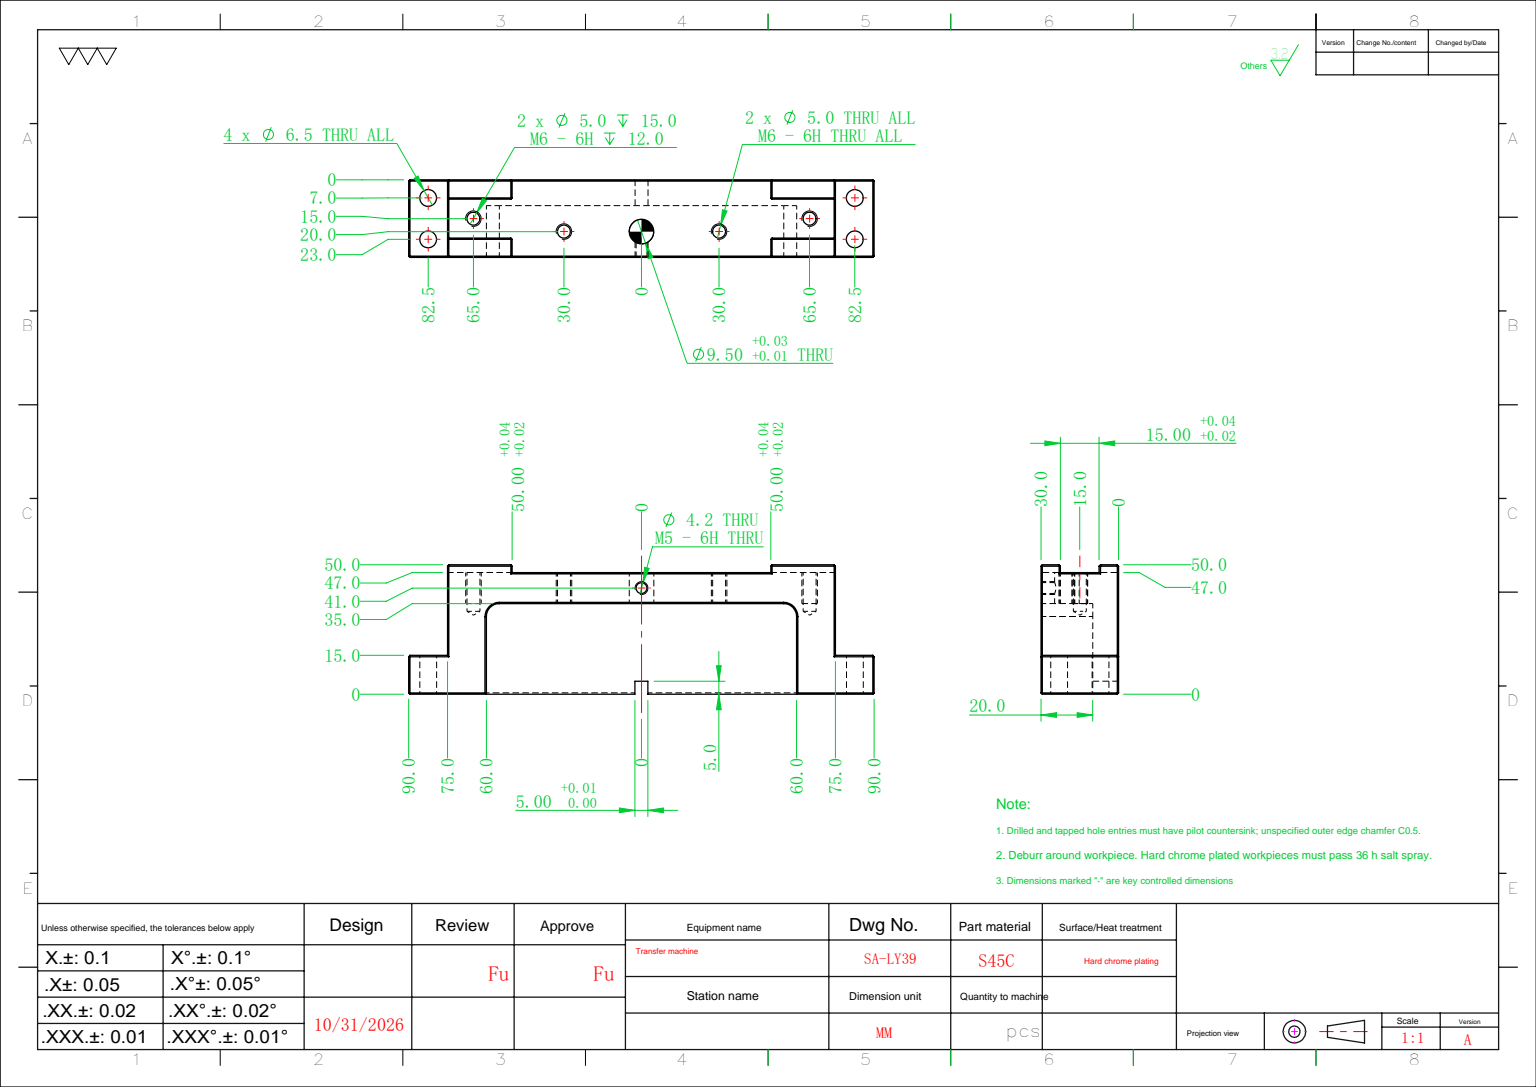
SolidWorks part; units mm, degrees
ref_plane "前视基准面" through (0, 0, 0) normal (0, 0, 1) x (1, 0, 0)
ref_plane "上视基准面" through (0, 0, 0) normal (0, 1, 0) x (1, 0, 0)
ref_plane "右视基准面" through (0, 0, 0) normal (1, 0, 0) x (0, 0, -1)
sketch "草图1" plane through (0, 0, 0) normal (0, 0, 1) x (1, 0, 0)
  line L1 (-75, -15) -> (75, -15)
  line L2 (-75, -15) -> (-75, 15)
  line L3 (-75, 15) -> (75, 15)
  line L4 (75, -15) -> (75, 15)
  line L5 (-75, -15) -> (75, 15) construction
  line L6 (-75, 15) -> (75, -15) construction
  point P0 (0, 0)
  dimension "D1" = 150
  dimension "D2" = 30
extrude "凸台-拉伸1" add sketch "草图1" along normal blind 50
sketch "草图3" plane through (0, -15, 0) normal (0, -1, 0) x (1, 0, 0)
  line L0 (-75, 50) -> (75, 50) construction
  line L1 (-60, 0) -> (60, 0)
  line L2 (-60, 0) -> (-60, 35)
  line L3 (-60, 35) -> (60, 35)
  line L4 (60, 0) -> (60, 35)
  line L5 (-75, 0) -> (75, 0) construction
  line L6 (0, 0) -> (0, 55.5607) construction
  dimension "D1" = 120
  dimension "D2" = 15
extrude "切除-拉伸2" cut sketch "草图3" against normal blind 20
sketch "草图4" plane through (0, -15, 0) normal (0, -1, 0) x (1, 0, 0)
  line L0 (-75, 50) -> (75, 50) construction
  line L1 (-50, 50) -> (50, 50)
  line L2 (-50, 50) -> (-50, 47)
  line L3 (-50, 47) -> (50, 47)
  line L4 (50, 50) -> (50, 47)
  line L5 (60, 35) -> (-60, 35) construction
  line L8 (0, 35) -> (0, 91.8101) construction
  dimension "D1" = 12
  dimension "D2" = 100
extrude "切除-拉伸3" cut sketch "草图4" against normal through all
sketch "草图5" plane through (0, 0, 50) normal (0, 0, 1) x (1, 0, 0)
  line L0 (-75, 15) -> (-75, -15) construction
  line L1 (-75, -7.5) -> (75, -7.5)
  line L2 (-75, -7.5) -> (-75, 7.5)
  line L3 (-75, 7.5) -> (75, 7.5)
  line L4 (75, -7.5) -> (75, 7.5)
  line L5 (75, -15) -> (75, 15) construction
  line L6 (0, 0) -> (95.2933, 0) construction
  dimension "D1" = 15
extrude "切除-拉伸4" cut sketch "草图5" against normal up to surface (3 mm away) up to face at (0, 0, 47)
fillet "圆角1" radius 5 2 edges at (-60, -5, 35) (60, -5, 35)
hole_wizard "M6 螺纹孔1" positions "草图9" profile "草图8" tap size "M6" standard "ISO" end condition through all
sketch "草图9" plane through (0, 0, 35) normal (0, 0, -1) x (-1, 0, 0)
  line L0 (0, 0) -> (0, -24.9786) construction
  line L2 (50, -15) -> (-50, -15) construction
  point P0 (30, -5)
  point P2 (-30, -5)
  dimension "D1" = 60
  dimension "D2" = 10
sketch "草图8" plane through (-30, -5, 35) normal (1, 0, 0) x (0, 1, 0)
  line L0 (0, 0) -> (0, 15)
  line L1 (0, 15) -> (2.5, 15)
  line L2 (2.5, 15) -> (2.5, 0)
  line L5 (2.5, 0) -> (0, 0)
  line L11 (0, -6.35) -> (0, 107.95) construction
  dimension "通孔螺纹孔钻头直径" = 5
  dimension "通孔螺纹孔钻头深度" = 15
cosmetic thread "孔螺蚊线1" parameters "D2"=6
cosmetic thread "孔螺蚊线2" parameters "D2"=6
sketch "草图11" plane through (0, 0, 35) normal (0, 0, -1) x (-1, 0, 0)
  line L0 (-30, -5) -> (30, -5) construction
  circle A0 centre (0, -5) radius 4.75
  dimension "D1" = 9.5
extrude "切除-拉伸6" cut sketch "草图11" against normal through all
hole_wizard "M5 螺纹孔1" positions "草图12" profile "草图13" tap size "M5" standard "ISO"
sketch "草图12" plane through (0, -15, 0) normal (0, -1, 0) x (-1, 0, 0)
  line L0 (0, -35) -> (0, -47) construction
  line L1 (-55, -35) -> (55, -35) construction
  line L2 (50, -47) -> (-50, -47) construction
  point P0 (0, -41)
sketch "草图13" plane through (0, -15, 41) normal (1, 0, 0) x (0, 0, -1)
  line L0 (0, 0) -> (0, 5.25)
  line L1 (0, 5.25) -> (2.1, 5.25)
  line L2 (2.1, 5.25) -> (2.1, 0)
  line L5 (2.1, 0) -> (0, 0)
  line L11 (0, -6.35) -> (0, 107.95) construction
  dimension "通孔螺纹孔钻头直径" = 4.2
  dimension "通孔螺纹孔钻头深度" = 5.25
cosmetic thread "孔螺蚊线3" parameters "D2"=5
hole_wizard "M6 螺纹孔2" positions "草图14" profile "草图15" tap size "M6" standard "ISO"
sketch "草图14" plane through (0, 0, 47) normal (0, 0, 1) x (1, 0, 0)
  line L0 (0, 0) -> (0, 33.0369) construction
  line L2 (0, 0) -> (95.1217, 0) construction
  point P0 (-65, 0)
  point P3 (65, 0)
  dimension "D1" = 130
sketch "草图15" plane through (-65, 0, 47) normal (1, 0, 0) x (0, -1, 0)
  line L0 (0, 0) -> (0, 16.5022)
  line L1 (0, 16.5022) -> (2.5, 15)
  line L2 (2.5, 15) -> (2.5, 0)
  line L5 (2.5, 0) -> (0, 0)
  line L10 (0, 16.5022) -> (-2.5, 15) construction
  line L11 (0, -6.35) -> (0, 107.95) construction
  dimension "螺纹孔钻头直径" = 5
  dimension "螺纹孔钻头深度" = 15
  dimension "导头角度" = 118
cosmetic thread "孔螺蚊线4" parameters "D1"=12, "D2"=6
cosmetic thread "孔螺蚊线5" parameters "D1"=12, "D2"=6
sketch "草图18" plane through (0, -15, 0) normal (0, -1, 0) x (1, 0, 0)
  line L0 (0, 0) -> (0, 48.8262) construction
  line L1 (-75, 0) -> (-90, 0)
  line L2 (-75, 0) -> (-75, 15)
  line L3 (-75, 15) -> (-90, 15)
  line L4 (-90, 0) -> (-90, 15)
  line L5 (90, 0) -> (90, 15)
  line L6 (75, 15) -> (90, 15)
  line L7 (75, 0) -> (75, 15)
  line L8 (75, 0) -> (90, 0)
  dimension "D1" = 15
  dimension "D2" = 15
extrude "凸台-拉伸2" add sketch "草图18" against normal up to surface (30 mm away) up to face at (0, 15, 36.75)
hole_wizard "Ø6.5 (6.5) 直径孔1" positions "草图19" profile "草图20" hole size "Ø6.5" standard "ISO" end condition through all
sketch "草图19" plane through (0, 0, 15) normal (0, 0, 1) x (1, 0, 0)
  line L0 (-90, 0) -> (90, 0) construction
  line L1 (-90, 15) -> (-90, -15) construction
  line L2 (90, 15) -> (90, -15) construction
  line L5 (0, 0) -> (0, -27.1316) construction
  point P0 (-82.5, 8)
  point P2 (-82.5, -8)
  point P23 (82.5, -8)
  point P24 (82.5, 8)
  dimension "D1" = 7.5
  dimension "D2" = 16
sketch "草图20" plane through (-82.5, 8, 15) normal (1, 0, 0) x (0, -1, 0)
  line L0 (0, 0) -> (0, 15)
  line L1 (0, 15) -> (3.25, 15)
  line L2 (3.25, 15) -> (3.25, 0)
  line L5 (3.25, 0) -> (0, 0)
  line L11 (0, -6.35) -> (0, 107.95) construction
  dimension "通孔孔直径" = 6.5
  dimension "通孔孔深度" = 15
sketch "草图21" plane through (0, 5, 0) normal (0, -1, 0) x (1, 0, 0)
  line L1 (-2.5, -5) -> (2.5, -5)
  line L2 (-2.5, -5) -> (-2.5, 5)
  line L3 (-2.5, 5) -> (2.5, 5)
  line L4 (2.5, -5) -> (2.5, 5)
  line L5 (-2.5, -5) -> (2.5, 5) construction
  line L6 (-2.5, 5) -> (2.5, -5) construction
  point P0 (0, 0)
  dimension "D1" = 5
  dimension "D2" = 10
extrude "切除-拉伸7" cut sketch "草图21" against normal through all
chamfer "倒角1" distance 0.5 angle 45 57 edges at (60, -15, 15) (-60, -15, 15) (58.5355, -15, 33.5355) (-58.5355, -15, 33.5355) (0, -15, 35) (90, 0, 0) (75, -15, 0) (90, 15, 7.5) (90, -15, 7.5) (90, 0, 15) (46.25, 15, 0) (-90, 0, 15) (-90, 15, 7.5) (-90, -15, 7.5) (-75, -15, 0) (-90, 0, 0) (-46.25, 15, 0) (0, -15, 47) (-50, -15, 48.5) (-50, -11.25, 50) (-50, -7.5, 48.5) (-62.5, -7.5, 50) (-62.5, 7.5, 50) (-50, 7.5, 48.5) (-50, 11.25, 50) (50, -11.25, 50) (50, -15, 48.5) (50, -7.5, 48.5) (50, 7.5, 48.5) (50, 11.25, 50) (62.5, 7.5, 50) (62.5, -7.5, 50) (82.5, 15, 15) (82.5, -15, 15) (75, -15, 32.5) (62.5, -15, 50) (75, -11.25, 50) (75, -7.5, 48.5) (75, 0, 47) (75, 7.5, 48.5) (75, 11.25, 50) (75, 15, 32.5) (62.5, 15, 50) (50, 15, 48.5) (0, 15, 47) (-50, 15, 48.5) (-62.5, 15, 50) (-82.5, 15, 15) (-82.5, -15, 15) (-75, 15, 32.5) (-75, 11.25, 50) (-75, 7.5, 48.5) (-75, 0, 47) (-75, -7.5, 48.5) (-62.5, -15, 50) (-75, -11.25, 50) (-75, -15, 32.5)
